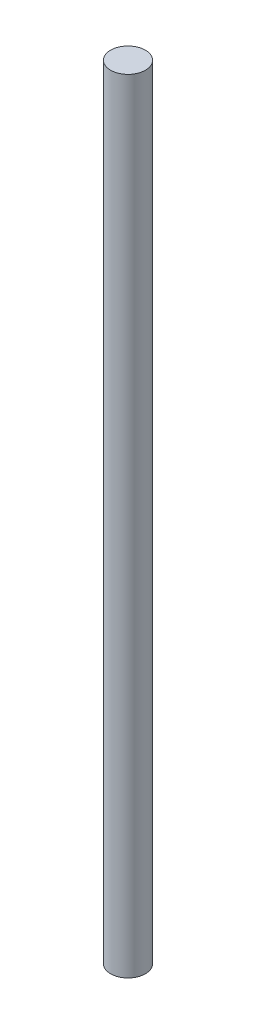
from build123d import *

# Parameters (mm, degrees)
SKETCH_1_R      = 4
EXTRUDE_1_DEPTH = 180


with BuildPart() as part:
    # 草图1 → 凸台-拉伸1 (new body)
    with BuildSketch(Plane(origin=(0, 0, 0), x_dir=(1, 0, 0), z_dir=(0, 1, 0))):
        with Locations(Location((0, 0, 0), (0, 0, 90))):
            Circle(SKETCH_1_R)
    extrude(amount=EXTRUDE_1_DEPTH)


solid = part.part
